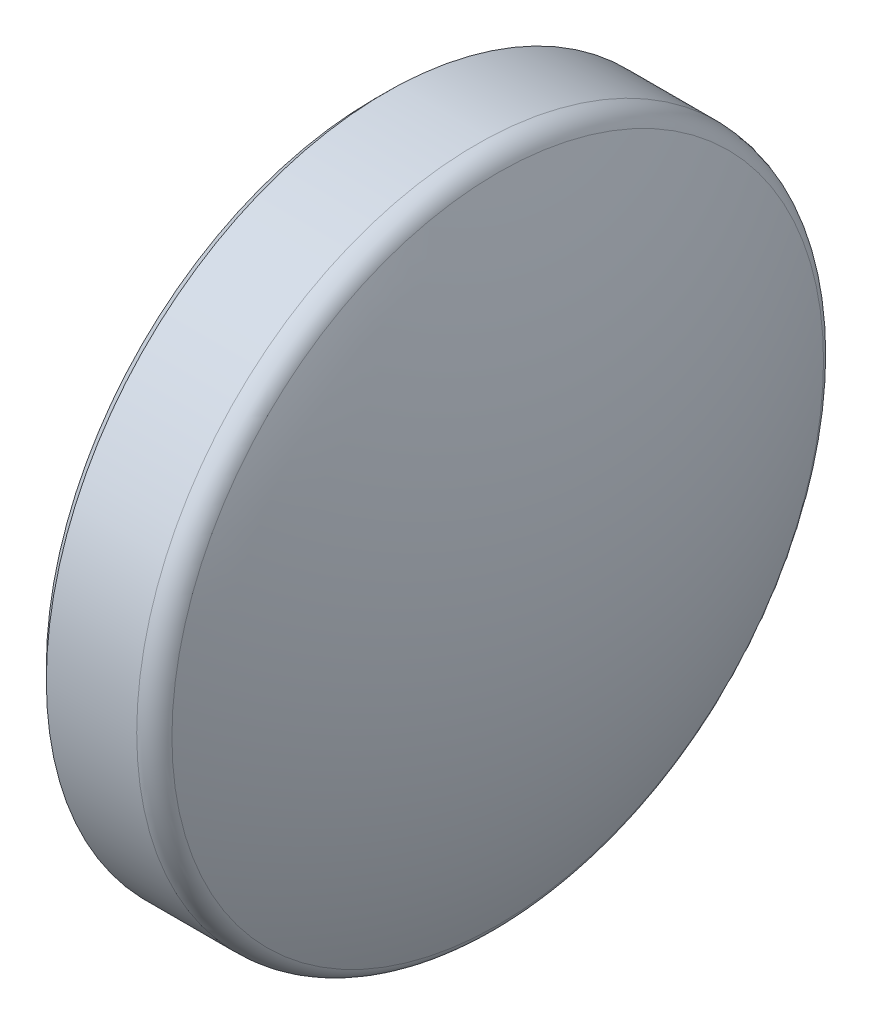
SolidWorks part; units mm, degrees
ref_plane "Front Plane" through (0, 0, 0) normal (0, 0, 1) x (1, 0, 0)
ref_plane "Top Plane" through (0, 0, 0) normal (0, 1, 0) x (1, 0, 0)
ref_plane "Right Plane" through (0, 0, 0) normal (1, 0, 0) x (0, 0, -1)
sketch "Sketch1" plane through (0, 0, 0) normal (0, 0, 1) x (1, 0, 0)
  line L0 (0, 0) -> (10, 0)
  line L2 (-110.5379, 29) -> (29.6555, 29) construction
  line L3 (0, 0) -> (0, 29)
  line L4 (0, 29) -> (16.4939, 29)
  arc A0 (10, 0) -> (16.4939, 29) centre (-51.5061, 29) ccw
  dimension "D1" = 68
  dimension "D4" = 29
  dimension "D2" = 10
revolve "Revolve1" add sketch "Sketch1" angle 360 about L2
fillet "Fillet2" radius 2 1 edges at (10, 29, 29)
chamfer "Chamfer1" distance 1 angle 45 1 edges at (0, 29, 29)
